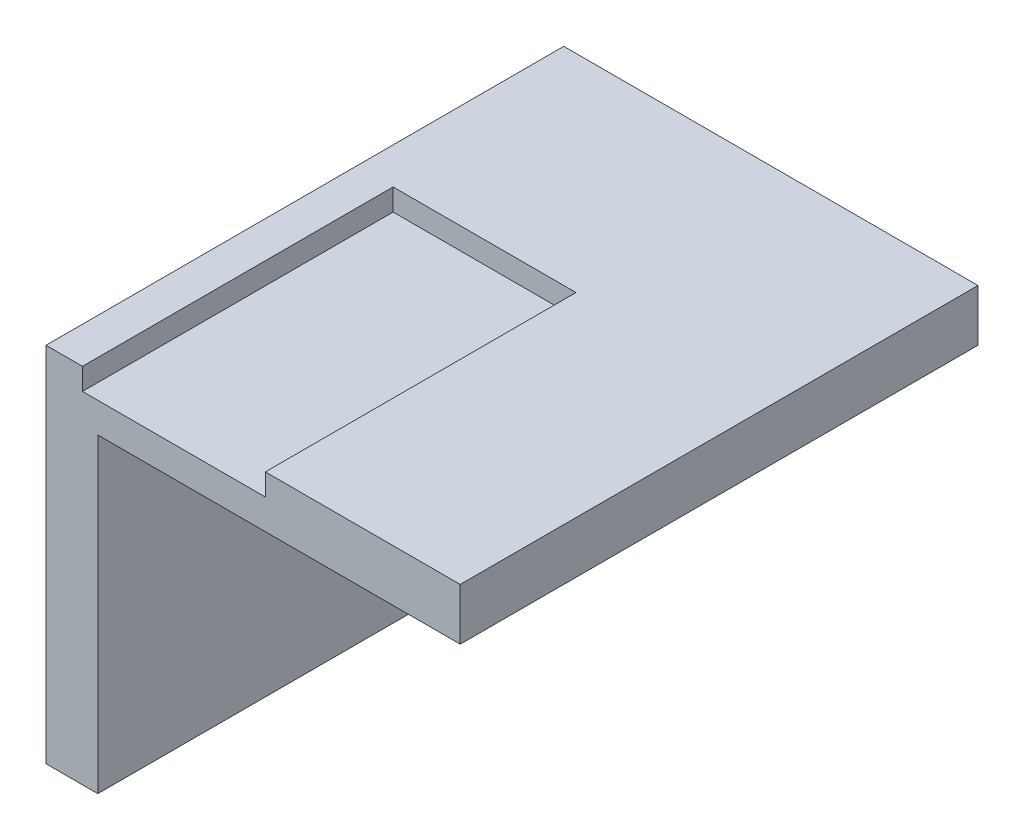
SolidWorks part; units mm, degrees
ref_plane "前视基准面" through (0, 0, 0) normal (0, 0, 1) x (1, 0, 0)
ref_plane "上视基准面" through (0, 0, 0) normal (0, 1, 0) x (1, 0, 0)
ref_plane "右视基准面" through (0, 0, 0) normal (1, 0, 0) x (0, 0, -1)
sketch "草图1" plane through (0, 0, 0) normal (0, 0, 1) x (1, 0, 0)
  line L0 (-37.5, 32.7885) -> (42.5, 32.7885)
  line L1 (42.5, 32.7885) -> (42.5, 22.7885)
  line L2 (42.5, 22.7885) -> (-27.5, 22.7885)
  line L3 (-27.5, 22.7885) -> (-27.5, -37.2115)
  line L4 (-27.5, -37.2115) -> (-37.5, -37.2115)
  line L5 (-37.5, -37.2115) -> (-37.5, 32.7885)
  dimension "D1" = 10
  dimension "D2" = 10
  dimension "D3" = 70
  dimension "D4" = 60
extrude "凸台-拉伸1" add sketch "草图1" along normal blind 100
sketch "草图2" plane through (0, 0, 100) normal (0, 0, 1) x (1, 0, 0)
  line L0 (-30.458, 32.7885) -> (-30.458, 28.5885)
  line L1 (42.5, 32.7885) -> (-37.5, 32.7885) construction
  line L2 (-30.458, 28.5885) -> (4.8599, 28.5885)
  line L3 (4.8599, 28.5885) -> (4.8599, 32.7885)
  line L4 (4.8599, 32.7885) -> (-30.458, 32.7885)
  dimension "D1" = 4.2
extrude "切除-拉伸1" cut sketch "草图2" against normal blind 60
